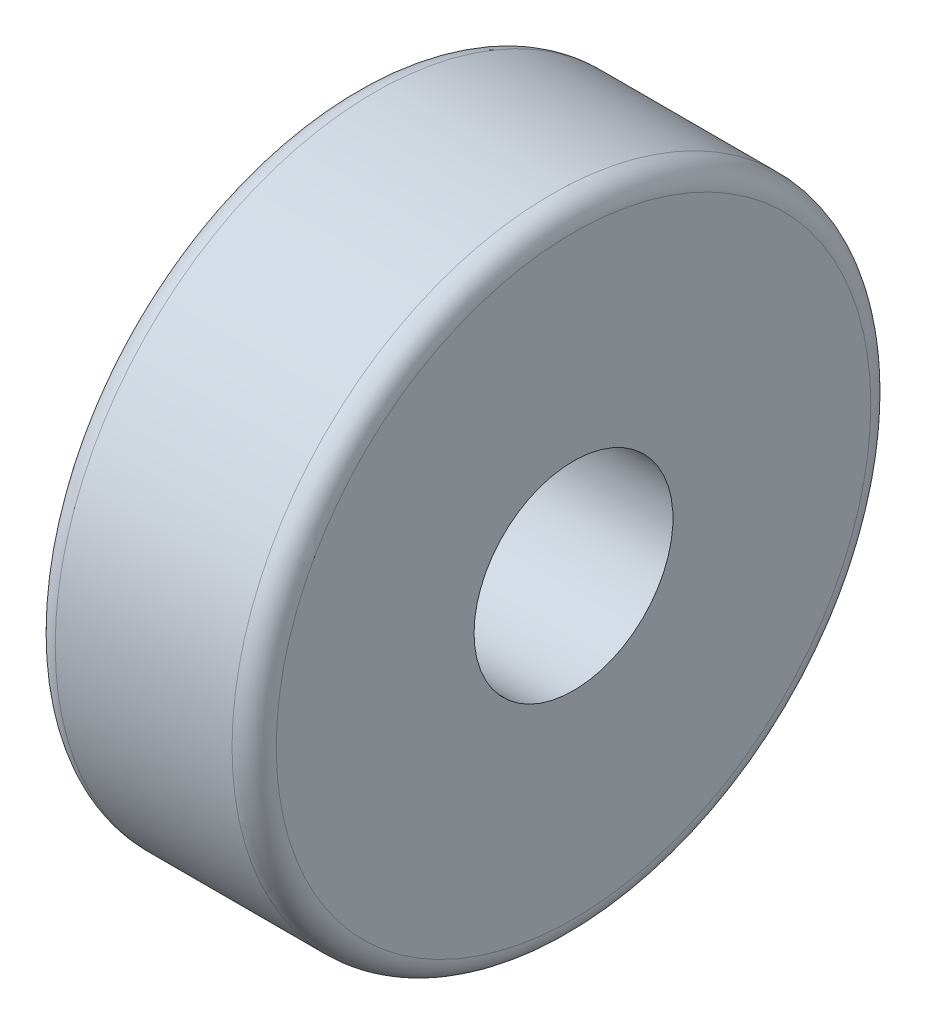
from build123d import *

# Parameters (mm, degrees)
SKETCH_1_W = 100
SKETCH_1_H = 99.5
FILLET_1_R = 10


with BuildPart() as part:
    # Sketch 1 → Revolve 1 (revolve)
    with BuildSketch(Plane.XY, mode=Mode.PRIVATE) as revolve_1_sk:
        with Locations((0, 94.75)):
            Rectangle(SKETCH_1_W, SKETCH_1_H)
    revolve(revolve_1_sk.sketch.rotate(Axis((-106.179775281, 0, 0), (1, 0, 0)), 90), axis=Axis((-106.179775281, 0, 0), (1, 0, 0)))

    # Fillet 1
    fillet_1_edges = [part.edges().sort_by_distance(p)[0] for p in [
        (50, 0, -144.5),
        (-50, 0, -144.5),
    ]]
    fillet(fillet_1_edges, radius=FILLET_1_R)


solid = part.part
